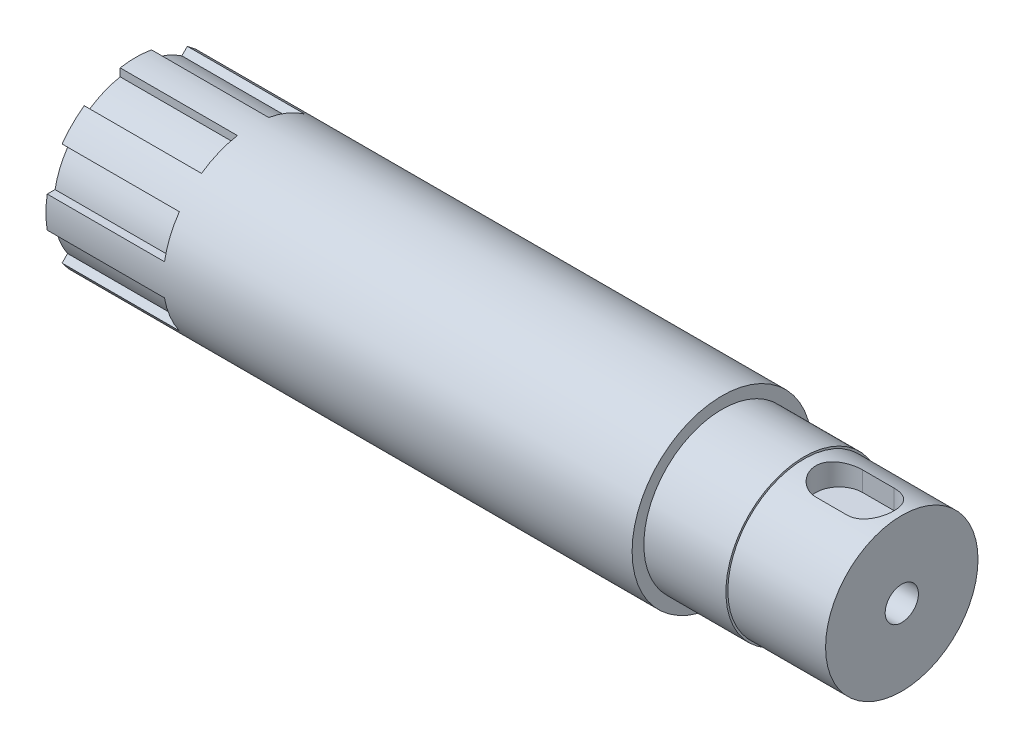
SolidWorks part; units mm, degrees
ref_plane "前视基准面" through (0, 0, 0) normal (0, 0, 1) x (1, 0, 0)
ref_plane "上视基准面" through (0, 0, 0) normal (0, 1, 0) x (1, 0, 0)
ref_plane "右视基准面" through (0, 0, 0) normal (1, 0, 0) x (0, 0, -1)
sketch "草图1" plane through (0, 0, 0) normal (1, 0, 0) x (0, 0, -1)
  circle A0 centre (0, 0) radius 19.5
extrude "凸台-拉伸1" add sketch "草图1" along normal blind 25
ref_plane "基准面1" through (0, 19.5, 0) normal (0, 1, 0) x (1, 0, 0)
sketch "草图2" plane through (0, 19.5, 0) normal (0, 1, 0) x (1, 0, 0)
  line L0 (9, 0) -> (17, 0) construction
  line L1 (9, 6) -> (17, 6)
  line L2 (9, -6) -> (17, -6)
  line L3 (25, -19.5) -> (25, 19.5) construction
  arc A0 (9, 6) -> (9, -6) centre (9, 0) ccw
  arc A1 (17, -6) -> (17, 6) centre (17, 0) ccw
  point P3 (13, 0)
  dimension "D1" = 6
  dimension "D3" = 8
  dimension "D2" = 8
extrude "切除-拉伸1" cut sketch "草图2" against normal blind 5.95
sketch "草图3" plane through (0, 0, 0) normal (-1, 0, 0) x (0, 0, 1)
  circle A0 centre (0, 0) radius 20
extrude "凸台-拉伸2" add sketch "草图3" along normal blind 21
sketch "草图4" plane through (-21, 0, 0) normal (-1, 0, 0) x (0, 0, 1)
  circle A0 centre (0, 0) radius 23
extrude "凸台-拉伸3" add sketch "草图4" along normal blind 150
sketch "草图5" plane through (-171, 0, 0) normal (-1, 0, 0) x (0, 0, 1)
  line L0 (0, 0) -> (0, 24.0401) construction
  line L2 (3.9848, 22.6522) -> (3.9848, 20.6522)
  line L4 (-4.0152, 20.6522) -> (-4.0152, 22.6468)
  line L7 (18.8352, 13.1998) -> (17.421, 11.7856)
  line L9 (11.7642, 17.4424) -> (13.1746, 18.8529)
  line L12 (22.6522, -3.9848) -> (20.6522, -3.9848)
  line L14 (20.6522, 4.0152) -> (22.6468, 4.0152)
  line L17 (13.1998, -18.8352) -> (11.7856, -17.421)
  line L19 (17.4424, -11.7642) -> (18.8529, -13.1746)
  line L22 (-3.9848, -22.6522) -> (-3.9848, -20.6522)
  line L24 (4.0152, -20.6522) -> (4.0152, -22.6468)
  line L27 (-18.8352, -13.1998) -> (-17.421, -11.7856)
  line L29 (-11.7642, -17.4424) -> (-13.1746, -18.8529)
  line L32 (-22.6522, 3.9848) -> (-20.6522, 3.9848)
  line L34 (-20.6522, -4.0152) -> (-22.6468, -4.0152)
  line L37 (-13.1998, 18.8352) -> (-11.7856, 17.421)
  line L39 (-17.4424, 11.7642) -> (-18.8529, 13.1746)
  circle A0 centre (0, 0) radius 23 construction
  arc A1 (-4.0152, 22.6468) -> (-13.1998, 18.8352) centre (0, 0) ccw
  arc A2 (-4.0152, 20.6522) -> (-11.7897, 17.4252) centre (0, 0) ccw
  arc A3 (11.7642, 17.4424) -> (3.9848, 20.658) centre (0, 0) ccw
  arc A4 (13.1746, 18.8529) -> (3.9848, 22.6522) centre (0, 0) ccw
  arc A5 (20.6522, 4.0152) -> (17.4252, 11.7897) centre (0, 0) ccw
  arc A6 (22.6468, 4.0152) -> (18.8352, 13.1998) centre (0, 0) ccw
  arc A7 (18.8529, -13.1746) -> (22.6522, -3.9848) centre (0, 0) ccw
  arc A8 (17.4424, -11.7642) -> (20.658, -3.9848) centre (0, 0) ccw
  arc A9 (4.0152, -22.6468) -> (13.1998, -18.8352) centre (0, 0) ccw
  arc A10 (4.0152, -20.6522) -> (11.7897, -17.4252) centre (0, 0) ccw
  arc A11 (-11.7642, -17.4424) -> (-3.9848, -20.658) centre (0, 0) ccw
  arc A12 (-13.1746, -18.8529) -> (-3.9848, -22.6522) centre (0, 0) ccw
  arc A13 (-22.6468, -4.0152) -> (-18.8352, -13.1998) centre (0, 0) ccw
  arc A14 (-20.6522, -4.0152) -> (-17.4252, -11.7897) centre (0, 0) ccw
  arc A15 (-17.4424, 11.7642) -> (-20.658, 3.9848) centre (0, 0) ccw
  arc A16 (-18.8529, 13.1746) -> (-22.6522, 3.9848) centre (0, 0) ccw
  point P48 (0, 0)
  circle M1 centre (0, 0) radius 23
  dimension "D1" = 8
extrude "切除-拉伸2" cut sketch "草图5" against normal blind 30 contours A8 L19 L12 M1 | A5 L14 L7 M1 | A14 L34 L27 M1 | A11 L29 L22 M1 | A10 L24 L17 M1 | A3 L9 L2 M1 | A2 L4 L37 M1 | A15 L39 L32 M1
hole_wizard "M10 螺纹孔1" positions "草图7" profile "草图6" tap size "M10" standard "Iso"
sketch "草图7" plane through (25, 0, 0) normal (1, 0, 0) x (0, 0, -1)
  point P0 (0, 0)
sketch "草图6" plane through (25, 0, 0) normal (0, 1, 0) x (0, 0, -1)
  line L0 (0, 0) -> (0, 22.5537)
  line L1 (0, 22.5537) -> (4.25, 20)
  line L2 (4.25, 20) -> (4.25, 0)
  line L5 (4.25, 0) -> (0, 0)
  line L10 (0, 22.5537) -> (-4.25, 20) construction
  line L11 (0, -6.35) -> (0, 107.95) construction
  dimension "螺纹孔钻头直径" = 8.5
  dimension "螺纹孔钻头深度" = 20
  dimension "导头角度" = 118
cosmetic thread "孔螺蚊线1"
